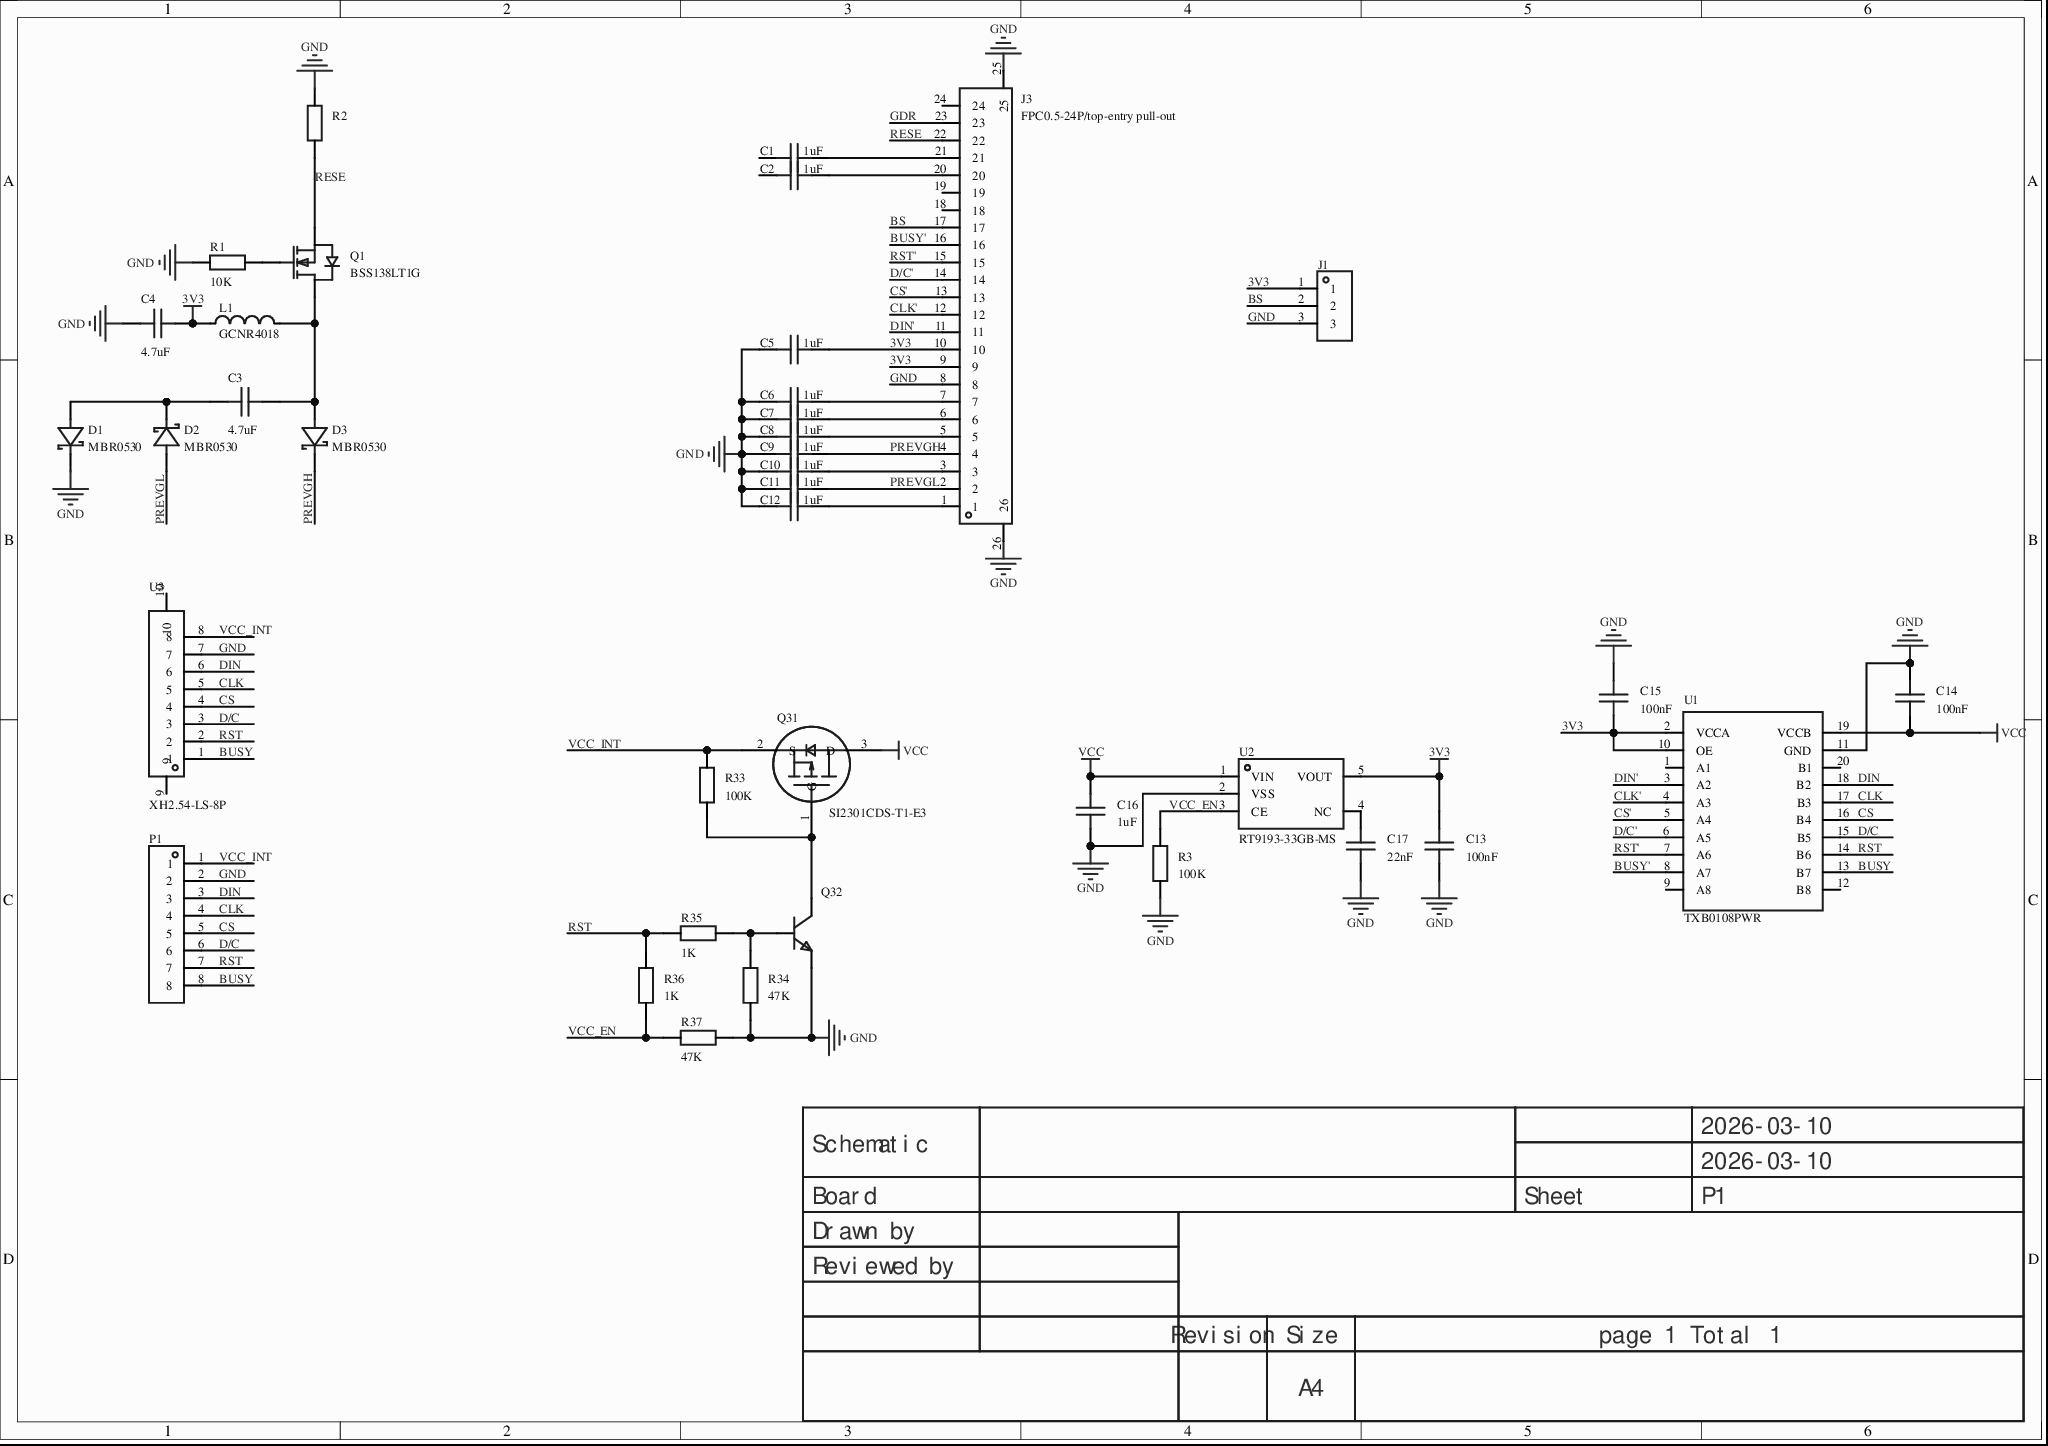
[diagram p0: MISC61435-3.schdoc]
# Altium project MISC61435-2.PrjPcb
1 sheet, 38 parts. Net scope: global (net labels, ports and power ports of the same name join across sheets).
Board file: MISC61435.pcbdoc

## Sheet MISC61435-3.schdoc
size 297 x 209 mm; Version: V1.0; @Project Name: MISC61435; @Update Date: 2026-03-10; @Create Date: 2026-03-10; @Board Name: MISC61435; @Create Time: 17:14:29; @Page Count: 1; @Page No: 1; @Schematic Name: MISC61435; @Update Time: 17:14:29; Size: A4

### Parts
C1  1uF  [C0603]
C2  1uF  [C0603]
C3  4.7uF  [C0603]
C4  4.7uF  [C0603]
C5  1uF  [C0603]
C6  1uF  [C0603]
C7  1uF  [C0603]
C8  1uF  [C0603]
C9  1uF  [C0603]
C10  1uF  [C0603]
C11  1uF  [C0603]
C12  1uF  [C0603]
C13  100nF  [C0603]
C14  100nF  [C0603]
C15  100nF  [C0603]
C16  1uF  [C0603]
C17  22nF  [C0603]
D1  MBR0530  [SOD-123FL_L2.7-W1.8-LS3.7-RD]
D2  MBR0530  [SOD-123FL_L2.7-W1.8-LS3.7-RD]
D3  MBR0530  [SOD-123FL_L2.7-W1.8-LS3.7-RD]
J1  (no value)  [HDR-TH_3P-P2.54-V-F]
J3  FPC0.5-24P/top-entry pull-out  [FPC-SMD_24P-P0.50_SHOU-HAN_CTSJ-H2.0]
L1  GCNR4018  [IND-SMD_L4.0-W4.0]
P1  (no value)  [HDR-TH_8P-P2.54-V-F-1]
Q1  BSS138LT1G  [SOT-23-3_L2.9-W1.6-P1.90-LS2.8-BR]
Q31  SI2301CDS-T1-E3  [SOT-23_L2.9-W1.3-P1.90-LS2.4-BR]
Q32  (no value)  [S8050_SOT-23]
R1  10K  [R0603]
R2  10K  [R0603]  (value not drawn)
R3  100K  [R0603]
R33  100K  [R0603]
R34  47K  [R0603]
R35  1K  [R0603]
R36  1K  [R0603]
R37  47K  [R0603]
U1  TXB0108PWR  [TSSOP-20_L6.5-W4.4-P0.65-LS6.4-BL]
U2  RT9193-33GB-MS  [SOT-23-5_L2.9-W1.6-P0.95-LS2.8-BR]
U3  XH2.54-LS-8P  [CONN-SMD_XH2.54-LS-8P]

### Nets
3V3: C4.2 C5.2 C13.2 C15.1 J1.1 J3.9 J3.10 L1.1 U1.2(VCCA) U1.10(OE) U2.5(VOUT)
GND: C4.1 C5.1 C6.1 C7.1 C8.1 C9.1 C10.1 C11.1 C12.1 C13.1 C14.2 C15.2 C16.1 C17.1 D1.1 J1.3 J3.8 J3.25 J3.26 P1.2 Q32.2 R1.2 R2.2 R3.1 R34.1 R37.2 U1.11(GND) U2.2(VSS) U3.7
VCC: C14.1 C16.2 Q31.3(D) U1.19(VCCB) U2.1(VIN)
BS: J1.2 J3.17
BUSY: P1.8 U1.13(B7) U3.1
BUSY': J3.16 U1.8(A7)
CLK: P1.4 U1.17(B3) U3.5
CLK': J3.12 U1.4(A3)
CS: P1.5 U1.16(B4) U3.4
CS': J3.13 U1.5(A4)
D/C: P1.6 U1.15(B5) U3.3
D/C': J3.14 U1.6(A5)
DIN: P1.3 U1.18(B2) U3.6
DIN': J3.11 U1.3(A2)
GDR: J3.23
PREVGH: C9.2 D3.1 J3.4
PREVGL: C11.2 D2.2 J3.2
RESE: J3.22 Q1.2(S) R2.1
RST: P1.7 R35.1 R36.2 U1.14(B6) U3.2
RST': J3.15 U1.7(A6)
VCC_EN: R3.2 R36.1 R37.1 U2.3(CE)
VCC_INT: P1.1 Q31.2(S) R33.2 U3.8
NetC1_2: C1.2 J3.21
NetC2_2: C2.2 J3.20
NetC3_1: C3.1 D1.2 D2.1
NetC3_2: C3.2 D3.2 L1.2 Q1.3(D)
NetC6_2: C6.2 J3.7
NetC7_2: C7.2 J3.6
NetC8_2: C8.2 J3.5
NetC10_2: C10.2 J3.3
NetC12_2: C12.2 J3.1
NetC17_2: C17.2 U2.4(NC)
NetQ1_1: Q1.1(G) R1.1
NetQ31_1: Q31.1(G) Q32.3 R33.1
NetQ32_1: Q32.1 R34.2 R35.2

Not connected (* = marked no-connect by the designer): C1 1; C2 1; J3 18 19 24; U1 1(A1) 9(A8) 12(B8) 20(B1); U3 9 10

### Notes on the sheet
- 2026-03-10
- Schematic
- Board
- Sheet
- P1
- Drawn by
- Reviewed by
- Revision
- Size
- A4
- page 1 Total 1

### Library data of the parts
C1-C17 = CAP_0603: Symbol: Capacitance; ConvertToPcb: yes; ModelId: ac125912035d415993ca9572d50418b10819f05c4eef4c71ace90d822a990e87; ModelName: C0603_L1.6-W0.8-H0.8; ModelTransform: 62.992,31.496,0,0,0,0,0,0,0; Device: CAP_0603; AddInBom: yes; Supplier Footprint: 0603; FootprintName: C0603
  C1 C2 C5-C12 C16: Value: 1uF
  C3 C4: Value: 4.7uF
  C13-C15: Value: 100nF
  C17: Value: 22nF
D1-D3 = MBR0530: Diode configuration: single; forward voltage (Vf): 550mV@500mA; DC reverse voltage (Vr): 30V; rectified current: 500mA;; Manufacturer: LGE(鲁光); Symbol: MBR0530_C2983233; AddInBom: yes; ModelId: 86f9151e155e4fe2af0c4f2e0a80302e0819f05c4eef4c71ace90d822a990e87; ModelName: SOD-123FL_L2.8-W1.8-H1.1-LS3.6; ModelTransform: 141.732,70.866,0,180,0,0,0,0,0; Reverse Leakage Current (Ir): 20uA@30V; Operating Junction Temperature Range: -55℃~+175℃; Non-Repetitive Peak Forward Surge Current: 15A; Device: MBR0530; LCSC Part Name: 电压:30V 电流:500mA; SupplierPart: C2983233; ManufacturerPart: MBR0530; Supplier Footprint: SOD-123FL; JLCPCB Part Class: Extended Part; Datasheet: https://example.com/datasheet/MBR0530/3419390.html; Supplier: LCSC; ConvertToPcb: yes; FootprintName: SOD-123FL_L2.7-W1.8-LS3.7-RD; Diode Configuration: Single; Voltage - Forward(Vf@If): 550mV@500mA; Voltage - DC Reverse(Vr): 30V; Current - Rectified: 500mA
J1 = HDR-F_2.54_1x3P: Symbol: PM254V-11-03-H85; ConvertToPcb: yes; ModelId: f3b3cc5aae9641bf9e56fc160cef875b0819f05c4eef4c71ace90d822a990e87; ModelName: HDR2.54-F-LI-1X3P; ModelTransform: 299.9994,100,0,0,0,0,0,0,-118.11; Device: HDR-F_2.54_1x3P; AddInBom: yes; SupplierPart: C541850; Supplier Footprint: 插件; FootprintName: HDR-TH_3P-P2.54-V-F
J3 = FPC0.5-24P/上接抽拉: AddInBom: yes; ModelId: 76a0ce5e92a64d6687145620a16e7ac30819f05c4eef4c71ace90d822a990e87; ModelTransform: 692.91204,208.661,0,0,0,0,0,-39.372,0; Symbol: FPC0.5-24P/top-entry pull-out; Device: FPC0.5-24P/top-entry pull-out; LCSC Part Name: FPC0.5-24P/上接抽拉; SupplierPart: C9900012923; ManufacturerPart: FPC0.5-24P/上接抽拉; Supplier Footprint: FPC-SMD_24P-P0.50_SHOU-HAN_CTSJ-H2.0; JLCPCB Part Class: Extended Part; Supplier: LCSC; ConvertToPcb: yes; FootprintName: FPC-SMD_24P-P0.50_SHOU-HAN_CTSJ-H2.0; ModelName: FPC-SMD_24P-P0.50_SHOU-HAN_CTSJ-H2.0
L1 = GCNR4018: AddInBom: yes; ModelId: 45bc3737ecfd4f3bb122605ee525b0180819f05c4eef4c71ace90d822a990e87; ModelName: IND-SMD_L4.0-W4.0-H1.9; ModelTransform: 157.48,157.484,0,0,0,0,0,0,0; Symbol: GCNR4018; Device: GCNR4018; LCSC Part Name: GCNR4018; SupplierPart: C9900001750; ManufacturerPart: GCNR4018; Supplier Footprint: 10uH用4.7uH代用; JLCPCB Part Class: Extended Part; Supplier: LCSC; ConvertToPcb: yes; FootprintName: IND-SMD_L4.0-W4.0
P1 = HDR-F_2.54_1x8P: Symbol: Header-Female-2.54_1x8; AddInBom: yes; ModelId: 0f7e4d9227ef4fa08d5469c22cc70cdb0819f05c4eef4c71ace90d822a990e87; ModelName: HDR-F-2.54_1x8; ModelTransform: 799.99844,100,0,0,0,0,0,0,-118.11; Device: HDR-F_2.54_1x8P; ConvertToPcb: yes; FootprintName: HDR-TH_8P-P2.54-V-F-1; SupplierPart: C27438; Supplier Footprint: 插件
Q1 = BSS138LT1G: Quantity: 1 N-channel; drain-source voltage (Vdss): 50V; continuous drain current (Id): 200mA; on-resistance (RDS(on)): 5.6Ω@2.75V; power dissipation (Pd): 225mW; threshold voltage (Vgs(th)): 500mV;; Manufacturer: onsemi(安森美); AddInBom: yes; ModelId: 89cb27a44ab2466697082bb9fd73a7d00819f05c4eef4c71ace90d822a990e87; ModelName: SOT-23-3L_L2.9-W1.6-H1.1-LS2.8-P0.95; ModelTransform: 114.173,110.236,0,90,0,0,0,0,0; Input Capacitance(Ciss): 50pF@25V; Reverse Transfer Capacitance (Crss@Vds): 5pF@25V; Symbol: BSS138LT1G; Device: BSS138LT1G; LCSC Part Name: 1个N沟道 耐压:50V 电流:200mA; SupplierPart: C82045; ManufacturerPart: BSS138LT1G; Supplier Footprint: SOT-23; JLCPCB Part Class: Extended Part; Datasheet: https://example.com/datasheet/BSS138LT1G/83200.html; Supplier: LCSC; ConvertToPcb: yes; FootprintName: SOT-23-3_L2.9-W1.6-P1.90-LS2.8-BR; Number: 1 N-channel; Drain to Source Voltage: 50V; Current - Continuous Drain(Id): 200mA; RDS(on): 5.6Ω@2.75V; Pd - Power Dissipation: 225mW; Gate Threshold Voltage (Vgs(th)): 500mV; Operating Temperature: -55℃~+150℃
Q31 = SI2301CDS-T1-E3: Quantity: 1 P-channel; drain-source voltage (Vdss): 20V; continuous drain current (Id): 3.1A; on-resistance (RDS(on)): 142mΩ@2.5V,2A; power dissipation (Pd): 1.6W; threshold voltage (Vgs(th)): 1V@250uA;; Manufacturer: VISHAY(威世); AddInBom: yes; ModelId: c62791f0466c4ae2a892c056b845b0ca0819f05c4eef4c71ace90d822a990e87; ModelName: SOT-23-3P_L2.9-W1.3-H1.0-LS2.4-P0.95; ModelTransform: 98.64468,114.173,0,180,0,0,0.001,-0.002,0; Input Capacitance(Ciss): 405pF; Reverse Transfer Capacitance (Crss@Vds): 55pF; Output Capacitance(Coss): 75pF; Symbol: SI2301CDS-T1-E3; Device: SI2301CDS-T1-E3; LCSC Part Name: 1个P沟道 耐压:20V 电流:3.1A; SupplierPart: C145226; ManufacturerPart: SI2301CDS-T1-E3; Supplier Footprint: SOT-23; JLCPCB Part Class: Extended Part; Datasheet: https://example.com/datasheet/SI2301CDS-T1-E3/156558.html; Supplier: LCSC; ConvertToPcb: yes; FootprintName: SOT-23_L2.9-W1.3-P1.90-LS2.4-BR; Number: 1 P-channel; Drain to Source Voltage: 20V; Current - Continuous Drain(Id): 3.1A; RDS(on): 142mΩ@2.5V,2A; Pd - Power Dissipation: 1.6W; Gate Threshold Voltage (Vgs(th)): 1V@250uA; Gate Charge(Qg): -; Operating Temperature: -55℃~+150℃; Type: P-channel
Q32 = S8050_SOT_NPN: Symbol: NPN; ConvertToPcb: yes; ModelId: c62791f0466c4ae2a892c056b845b0ca0819f05c4eef4c71ace90d822a990e87; ModelName: SOT-23-3P_L2.9-W1.3-H1.0-LS2.4-P0.95; ModelTransform: 98.6,114.12,41.29,180,0,0,0,0,-3; Device: S8050_SOT_NPN; AddInBom: yes; Supplier Footprint: SOT-23; FootprintName: S8050_SOT-23
R1-R3 R33-R37 = Res_0603: Symbol: Resistor; ConvertToPcb: yes; ModelId: fc143cca1e79419f9cd78b61e9279f080819f05c4eef4c71ace90d822a990e87; ModelTransform: 31.8897,63.7794,0,90,0,0,0,0,0; Device: Res_0603; AddInBom: yes; Supplier Footprint: 0603; FootprintName: R0603; ModelName: R0603
  R1 R2: Value: 10K
  R3 R33: Value: 100K
  R34 R37: Value: 47K
  R35 R36: Value: 1K
U1 = TXB0108PWR: Data rate: 100Mbps; voltage (VCCA): 1.2V~3.6V; voltage (VCCB): 1.65V~5.5V; number of circuits: 1; channels per circuit: 8;; Manufacturer: TI(德州仪器); AddInBom: yes; ModelId: c491f68934b34c649df5890a1d97cd0f0819f05c4eef4c71ace90d822a990e87; ModelName: TSSOP-20_L6.5-W4.4-H1.0-LS6.4-P0.65; ModelTransform: 251.969,255.906,0,90,0,0,0.0005,0,0; Channel Type: Bidirectional; Number of Circuits: 1; Channels per Circuit: 8; Output Type: Tri-state; non-inverting; Symbol: TXB0108PWR; Device: TXB0108PWR; LCSC Part Name: 100Mbps 8位双向电平转换器; SupplierPart: C53406; ManufacturerPart: TXB0108PWR; Supplier Footprint: TSSOP-20; JLCPCB Part Class: Extended Part; Supplier: LCSC; ConvertToPcb: yes; FootprintName: TSSOP-20_L6.5-W4.4-P0.65-LS6.4-BL; Input Signal: -; Output Signal: -; Data Rate: 100Mbps; Supply Voltage (VCCA): 1.2V~3.6V; Supply Voltage (VCCB): 1.65V~5.5V; Operating Temperature: -40℃~+85℃; Features: Automatic direction sensing
U2 = RT9193-33GB-MS: Output type: fixed; max input voltage: 6V; output voltage: 3.3V; max output current: 300mA; power supply ripple rejection (PSRR): 70dB@(1kHz); output polarity: positive;; Manufacturer: MSKSEMI(美森科); AddInBom: yes; ModelId: 7ba65df16e7b4570af156e925f9c37fe0819f05c4eef4c71ace90d822a990e87; ModelTransform: 114.173,114.173,0,90,0,0,0,0,0; standby current: 70uA; Symbol: RT9193-33GB-MS; Device: RT9193-33GB-MS; LCSC Part Name: RT9193-33GB-MS; SupplierPart: C7528825; ManufacturerPart: RT9193-33GB-MS; Supplier Footprint: SOT-23-5; JLCPCB Part Class: Extended Part; Datasheet: https://example.com/upload/public/pdf/source/20230821/D8074B49A3EB388F72C6079FFA866DDB.pdf; Supplier: LCSC; ConvertToPcb: yes; FootprintName: SOT-23-5_L2.9-W1.6-P0.95-LS2.8-BR; ModelName: SOT-23-5_L2.9-W1.6-P0.95-LS2.8-BR; Output Type: Fixed; Maximum Input Voltage: 6V; Output Voltage: 3.3V; MAX Output Current: 300mA; Power Supply Rejection Ratio (PSRR): 70dB@(1kHz); Output Polarity: Positive
U3 = XH2.54-LS-8P: AddInBom: yes; ModelId: 30cda136a516485b8f27b800c7ecc17c0819f05c4eef4c71ace90d822a990e87; ModelTransform: 984.25,330.708,0,0,0,0,0,8.74,0; Symbol: XH2.54-LS-8P; Device: XH2.54-LS-8P; LCSC Part Name: XH2.54-LS-8P; SupplierPart: C9900010308; ManufacturerPart: XH2.54-LS-8P; Supplier Footprint: HA-08ASMT-T3R(H); JLCPCB Part Class: Extended Part; Supplier: LCSC; ConvertToPcb: yes; FootprintName: CONN-SMD_XH2.54-LS-8P; ModelName: CONN-SMD_XH2.54-LS-8P